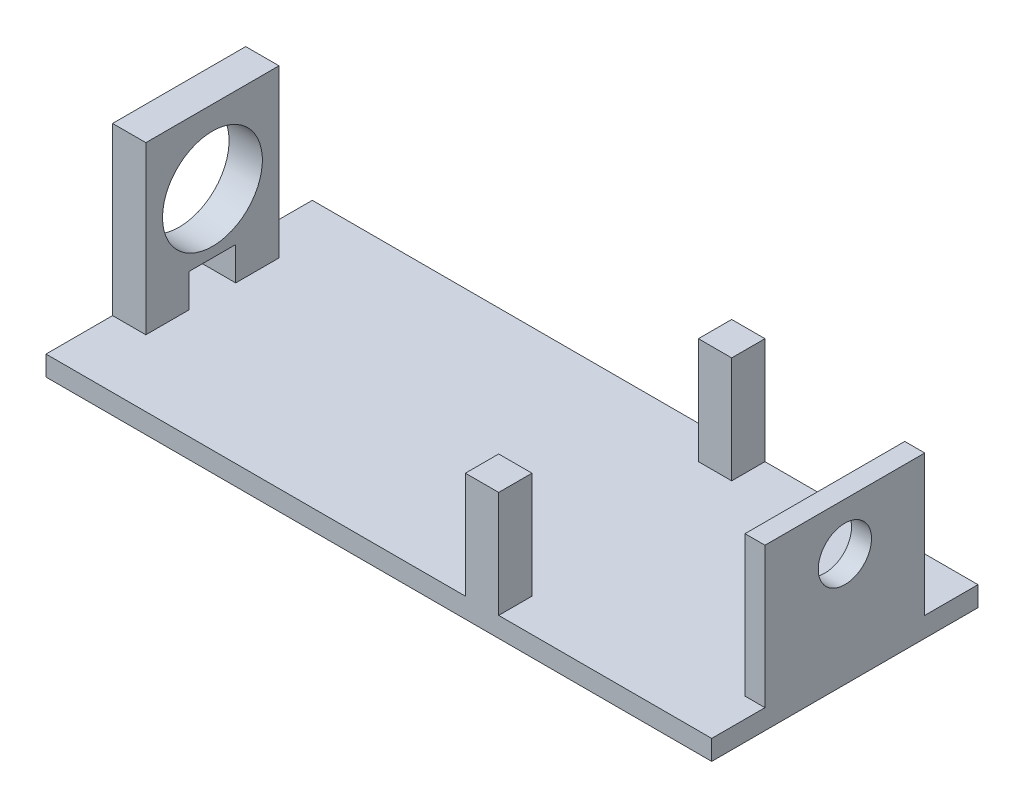
SolidWorks part; units mm, degrees
ref_plane "Front Plane" through (0, 0, 0) normal (0, 0, 1) x (1, 0, 0)
ref_plane "Top Plane" through (0, 0, 0) normal (0, 1, 0) x (1, 0, 0)
ref_plane "Right Plane" through (0, 0, 0) normal (1, 0, 0) x (0, 0, -1)
sketch "Sketch1" plane through (0, 0, 0) normal (0, 1, 0) x (1, 0, 0)
  line L1 (-50, -20) -> (50, -20)
  line L2 (-50, -20) -> (-50, 20)
  line L3 (-50, 20) -> (50, 20)
  line L4 (50, -20) -> (50, 20)
  line L5 (-50, -20) -> (50, 20) construction
  line L6 (-50, 20) -> (50, -20) construction
  point P0 (0, 0)
  dimension "D1" = 40
  dimension "D2" = 100
extrude "Boss-Extrude1" add sketch "Sketch1" along normal blind 3
ref_plane "Plane1" through (40, 0, 0) normal (1, 0, 0) x (0, 0, -1)
sketch "Sketch2" plane through (40, 0, 0) normal (1, 0, 0) x (0, 0, -1)
  line L0 (-10, 3) -> (-10, 28)
  line L1 (-20, 3) -> (20, 3) construction
  line L2 (-10, 28) -> (10, 28)
  line L3 (10, 28) -> (10, 3)
  line L4 (10, 3) -> (-10, 3)
  circle A0 centre (0, 17) radius 7.5
  dimension "D3" = 15
  dimension "D1" = 10
  dimension "D2" = 20
  dimension "D4" = 14
  dimension "D5" = 25
extrude "Boss-Extrude2" add sketch "Sketch2" along normal blind 5
sketch "Sketch3" plane through (-50, 0, 0) normal (-1, 0, 0) x (0, 0, 1)
  line L4 (-10, 3) -> (10, 3)
  line L5 (10, 3) -> (10, 28)
  line L6 (10, 28) -> (-10, 28)
  line L7 (-10, 28) -> (-10, 3)
  line L8 (-10, 3) -> (-3.5, 3)
  line L9 (10, 3) -> (10, 28)
  line L10 (10, 28) -> (-10, 28)
  line L11 (-10, 28) -> (-10, 3)
  line L12 (10, 3) -> (3.5, 3)
  line L13 (-3.5, 3) -> (-3.5, 8)
  line L14 (-3.5, 8) -> (3.5, 8)
  line L15 (3.5, 8) -> (3.5, 3)
  circle A0 centre (0, 17) radius 7.5 construction
  circle A1 centre (0, 17) radius 7.5
  dimension "D2" = 5
  dimension "D3" = 7
  dimension "D4" = 3.5
  dimension "D1" = 0
extrude "Boss-Extrude3" add sketch "Sketch3" against normal blind 5
ref_plane "Plane2" through (13, 0, 0) normal (1, 0, 0) x (0, 0, -1)
sketch "Sketch4" plane through (13, 0, 0) normal (1, 0, 0) x (0, 0, -1)
  line L5 (20, 3) -> (15, 3)
  line L6 (20, 3) -> (20, 19)
  line L7 (20, 19) -> (15, 19)
  line L13 (15, 3) -> (15, 19)
  line L14 (-20, 3) -> (-15, 3)
  line L18 (-20, 3) -> (-20, 19)
  line L19 (-20, 19) -> (-15, 19)
  line L21 (-15, 3) -> (-15, 19)
  dimension "D3" = 16
  dimension "D4" = 16
  dimension "D1" = 5
  dimension "D2" = 5
extrude "Boss-Extrude4" add sketch "Sketch4" along normal blind 5
sketch "Sketch7" plane through (50, 0, 0) normal (1, 0, 0) x (0, 0, -1)
  line L0 (-12, 0) -> (-12, 24.1317)
  line L1 (-20, 0) -> (20, 0) construction
  line L2 (-12, 24.1317) -> (12, 24.1317)
  line L3 (12, 24.1317) -> (12, 0)
  line L4 (12, 0) -> (-12, 0)
  circle A0 centre (0, 17) radius 4
  dimension "D3" = 8
  dimension "D1" = 24
  dimension "D2" = 12
extrude "Boss-Extrude5" add sketch "Sketch7" against normal blind 3
sketch "Sketch9" plane through (0, 3, 0) normal (0, 1, 0) x (1, 0, 0)
  line L1 (45.2042, -11.4602) -> (36.2907, -11.4602)
  line L2 (45.2042, -11.4602) -> (45.2042, 11.4602)
  line L3 (45.2042, 11.4602) -> (36.2907, 11.4602)
  line L4 (36.2907, -11.4602) -> (36.2907, 11.4602)
extrude "Cut-Extrude3" cut sketch "Sketch9" along normal blind 47
